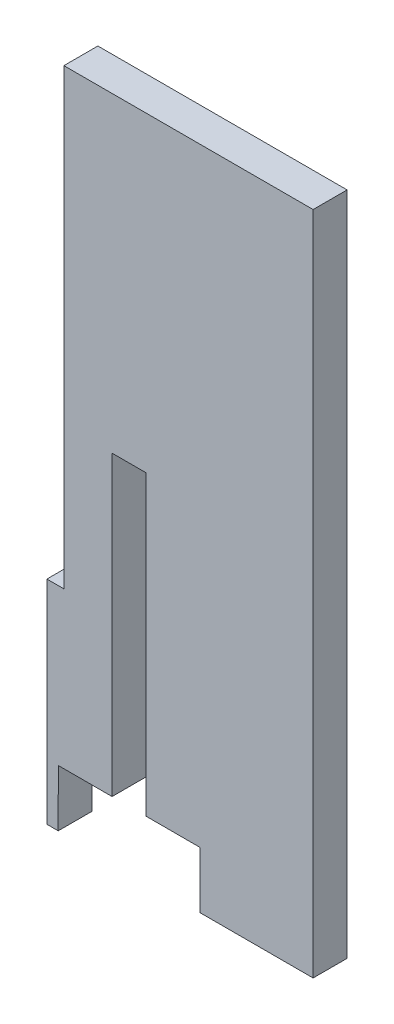
SolidWorks part; units mm, degrees
material "Q235B"
ref_plane "Front Plane" through (0, 0, 0) normal (0, 0, 1) x (1, 0, 0)
ref_plane "Top Plane" through (0, 0, 0) normal (0, 1, 0) x (1, 0, 0)
ref_plane "Right Plane" through (0, 0, 0) normal (1, 0, 0) x (0, 0, -1)
sketch "Sketch1" plane through (0, 0, 0) normal (0, 0, 1) x (1, 0, 0)
  line L0 (127.0127, -33.4453) -> (107.0127, -33.4453)
  line L2 (107.0127, -33.4453) -> (107.0127, 84.0547)
  line L4 (127.0127, -33.4453) -> (127.0206, -23.4453)
  line L6 (152.0145, -33.4453) -> (172.0145, -33.4453)
  line L7 (172.0145, -33.4453) -> (172.0145, 84.0547)
  line L8 (172.0145, 84.0547) -> (107.0127, 84.0547)
  line L9 (127.0206, -23.4453) -> (152.0224, -23.4651)
  line L10 (152.0224, -23.4651) -> (152.0145, -33.4453)
  dimension "D1" = 20
  dimension "D2" = 25.0018
  dimension "D3" = 20
  dimension "D4" = 117.5
extrude "Boss-Extrude1" add sketch "Sketch1" along normal blind 6
sketch "Sketch3" plane through (0, 0, 0) normal (0, 0, -1) x (-1, 0, 0)
  line L0 (-142.5165, 29.0547) -> (-142.5165, -30.9453)
  line L1 (-142.5165, 29.0547) -> (-136.5165, 29.0547)
  line L2 (-136.5165, 29.0547) -> (-136.5165, -30.9453)
  line L3 (-142.5165, -30.9453) -> (-136.5165, -30.9453)
  line L4 (-152.0224, -23.4651) -> (-152.0145, -33.4453) construction
  line L5 (-172.0145, 84.0547) -> (-107.0127, 84.0547) construction
  point P2 (-139.5165, -30.9453)
  dimension "D2" = 12.5
  dimension "D3" = 55
  dimension "D4" = 60
  dimension "D1" = 6
extrude "Cut-Extrude1" cut sketch "Sketch3" against normal blind 10
sketch "Sketch4" plane through (0, 0, 6) normal (0, 0, 1) x (1, 0, 0)
  line L1 (125.0127, -36.5804) -> (107.0127, -36.5804)
  line L2 (107.0127, 84.0547) -> (107.0127, -33.4453) construction
  line L3 (107.0127, -36.5804) -> (107.0127, 84.0547)
  line L4 (107.0127, 84.0547) -> (128.0127, 84.0547)
  line L5 (172.0145, 84.0547) -> (107.0127, 84.0547) construction
  line L6 (125.0127, 4.0547) -> (125.0127, -36.5804)
  line L7 (125.0127, 4.0547) -> (128.0127, 4.0547)
  line L8 (128.0127, 4.0547) -> (128.0127, 84.0547)
  line L9 (172.0145, 84.0547) -> (107.0127, 84.0547) construction
  dimension "D1" = 21
  dimension "D2" = 3
  dimension "D3" = 80
extrude "Cut-Extrude2" cut sketch "Sketch4" against normal through all
